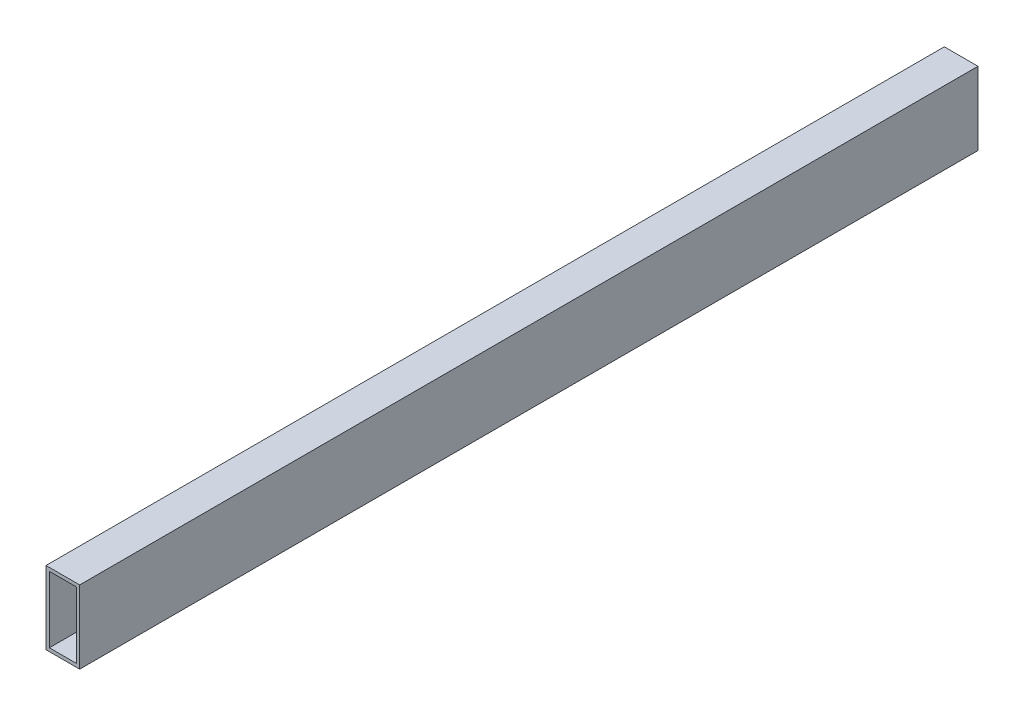
from build123d import *

# Parameters (mm, degrees)
SKETCH1_W           = 30
SKETCH1_H           = 65
BOSS_EXTRUDE1_DEPTH = 800
CUT_EXTRUDE1_DEPTH  = 800


with BuildPart() as part:
    # Sketch1 → Boss-Extrude1 (new body)
    with BuildSketch(Plane.XY):
        with Locations((-25.852518101, 6.473439942)):
            Rectangle(SKETCH1_W, SKETCH1_H)
    extrude(amount=BOSS_EXTRUDE1_DEPTH)

    # Sketch2 → Cut-Extrude1 (cut)
    with BuildSketch(Plane.XY.offset(800)):
        Polygon((-37.852518101, 35.207148711), (-37.852518101, -23.026560058), (-13.852518101, -23.026560058), (-13.852518101, 35.973439942), (-37.852518101, 35.973439942), align=None)
    extrude(amount=-CUT_EXTRUDE1_DEPTH, mode=Mode.SUBTRACT)


solid = part.part
